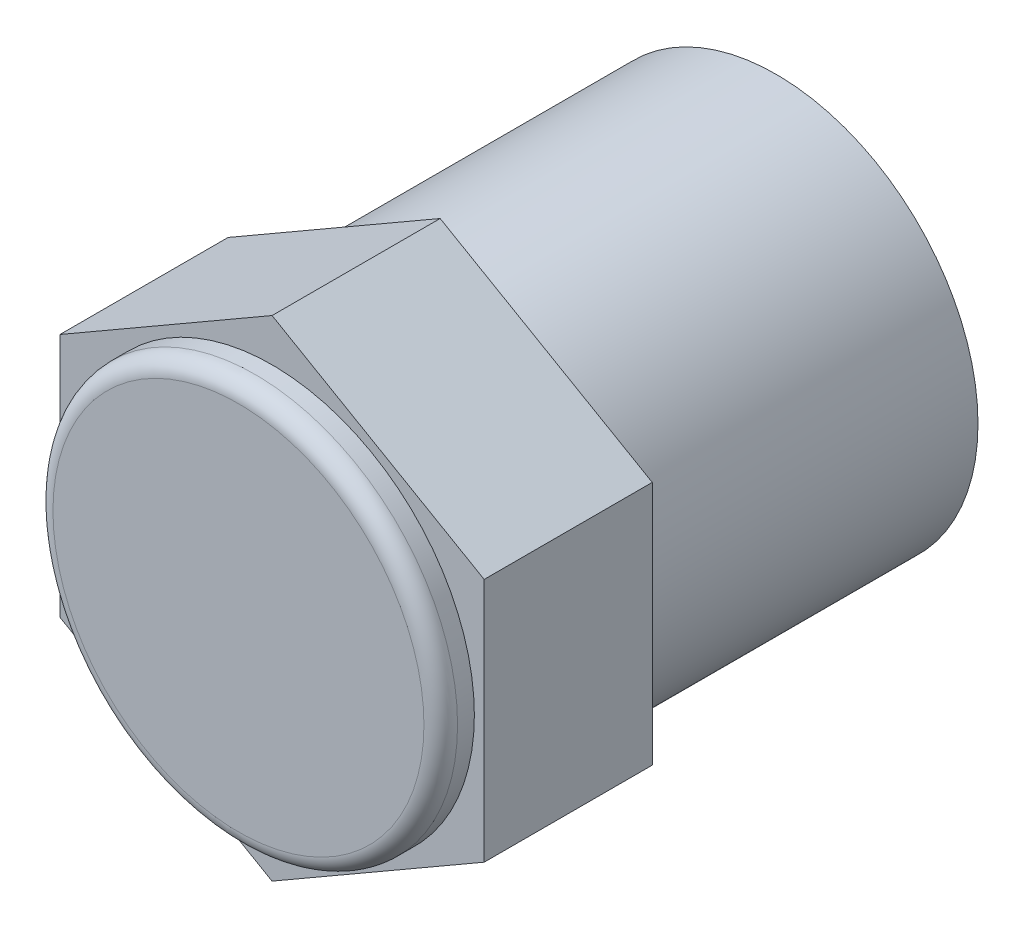
SolidWorks part; units mm, degrees
ref_plane "Front Plane" through (0, 0, 0) normal (0, 0, 1) x (1, 0, 0)
ref_plane "Top Plane" through (0, 0, 0) normal (0, 1, 0) x (1, 0, 0)
ref_plane "Right Plane" through (0, 0, 0) normal (1, 0, 0) x (0, 0, -1)
sketch "Sketch1" plane through (0, 0, 0) normal (0, 0, 1) x (1, 0, 0)
  circle A0 centre (0, 0) radius 6
extrude "Boss-Extrude1" add sketch "Sketch1" along normal blind 10
sketch "Sketch2" plane through (0, 0, 10) normal (0, 0, 1) x (1, 0, 0)
  line L1 (0, 7.2858) -> (-6.3097, 3.6429)
  line L2 (-6.3097, 3.6429) -> (-6.3097, -3.6429)
  line L3 (-6.3097, -3.6429) -> (0, -7.2858)
  line L4 (0, -7.2858) -> (6.3097, -3.6429)
  line L5 (6.3097, -3.6429) -> (6.3097, 3.6429)
  line L6 (6.3097, 3.6429) -> (0, 7.2858)
  circle A0 centre (0, 0) radius 6.3097 construction
extrude "Boss-Extrude2" add sketch "Sketch2" along normal blind 5
sketch "Sketch3" plane through (0, 0, 15) normal (0, 0, 1) x (1, 0, 0)
  circle A0 centre (0, 0) radius 6.018
extrude "Boss-Extrude3" add sketch "Sketch3" along normal blind 1
fillet "Fillet2" radius 0.5 1 edges at (6.018, 0, 16)
